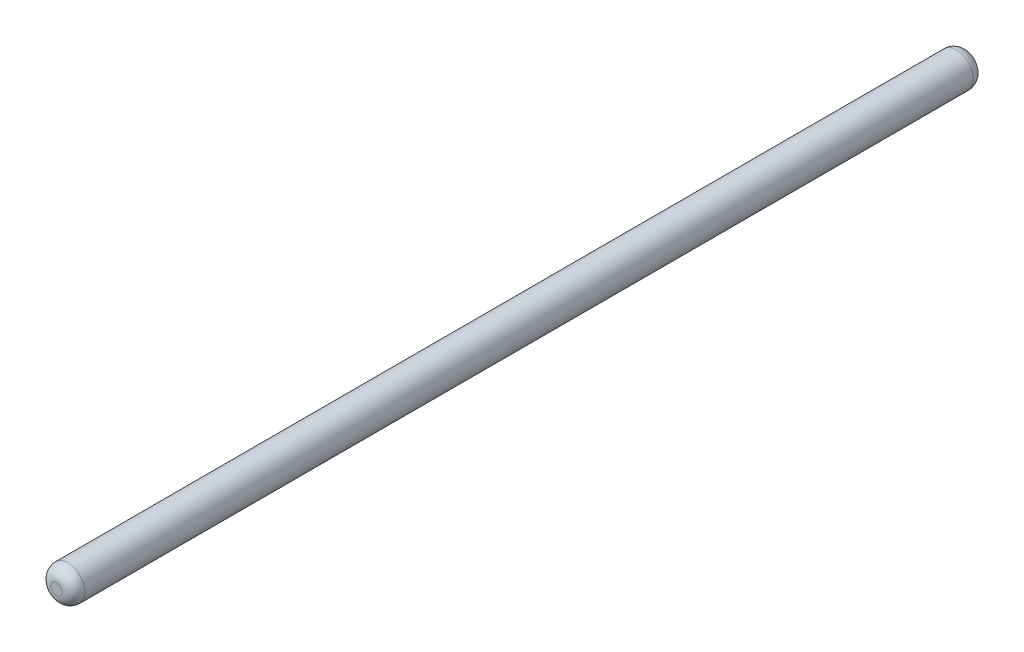
SolidWorks part; units mm, degrees
ref_plane "Front Plane" through (0, 0, 0) normal (0, 0, 1) x (1, 0, 0)
ref_plane "Top Plane" through (0, 0, 0) normal (0, 1, 0) x (1, 0, 0)
ref_plane "Right Plane" through (0, 0, 0) normal (1, 0, 0) x (0, 0, -1)
other "Configuration Table"
sketch "Sketch1" plane through (0, 0, 0) normal (0, 0, 1) x (1, 0, 0)
  circle A0 centre (0, 0) radius 0.75
  dimension "D1" = 1.5
extrude "Boss-Extrude1" add sketch "Sketch1" along normal blind 40 contours A0
fillet "Fillet1" radius 0.5 2 edges at (0.75, 0, 40) (0.75, 0, 0)
